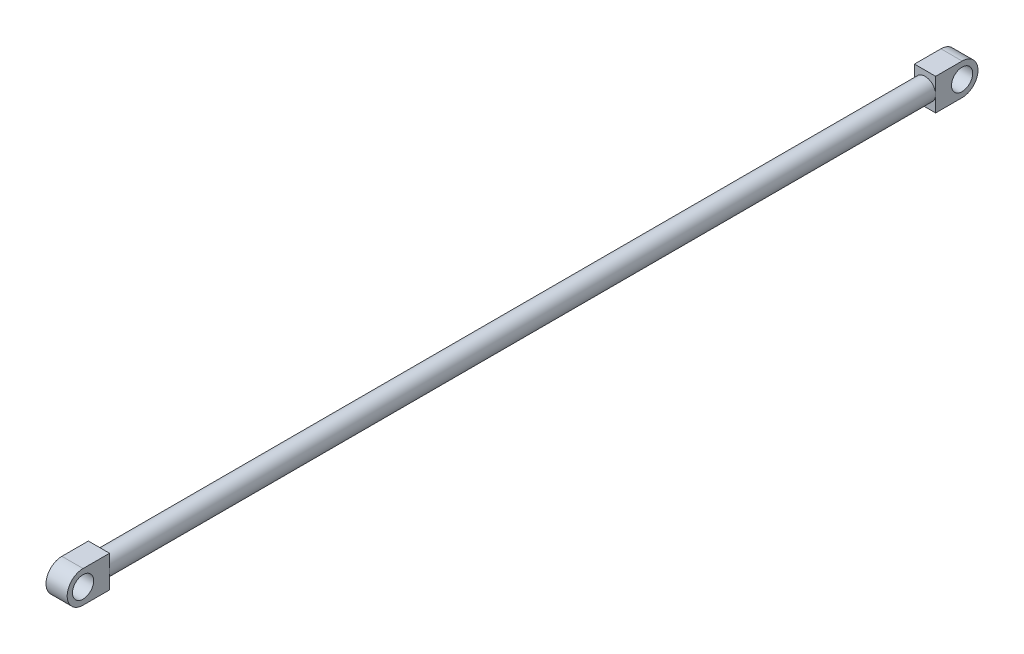
SolidWorks part; units mm, degrees
ref_plane "Front Plane" through (0, 0, 0) normal (0, 0, 1) x (1, 0, 0)
ref_plane "Top Plane" through (0, 0, 0) normal (0, 1, 0) x (1, 0, 0)
ref_plane "Right Plane" through (0, 0, 0) normal (1, 0, 0) x (0, 0, -1)
other "Configuration Table"
sketch "Sketch1" plane through (0, 0, 0) normal (0, 0, 1) x (1, 0, 0)
  circle A0 centre (0, 0) radius 5
  dimension "D1" = 10
extrude "Boss-Extrude1" add sketch "Sketch1" along normal blind 390
sketch "Sketch2" plane through (0, 0, 0) normal (0, 0, -1) x (-1, 0, 0)
  line L1 (-5, 7.5) -> (5, 7.5)
  line L2 (-5, 7.5) -> (-5, -7.5)
  line L3 (-5, -7.5) -> (5, -7.5)
  line L4 (5, 7.5) -> (5, -7.5)
  line L5 (-5, 7.5) -> (5, -7.5) construction
  line L6 (-5, -7.5) -> (5, 7.5) construction
  point P0 (0, 0)
  dimension "D1" = 10
  dimension "D2" = 15
extrude "Boss-Extrude2" add sketch "Sketch2" along normal blind 20
sketch "Sketch3" plane through (0, 0, 390) normal (0, 0, 1) x (1, 0, 0)
  line L1 (-5, -7.5) -> (5, -7.5)
  line L2 (-5, -7.5) -> (-5, 7.5)
  line L3 (-5, 7.5) -> (5, 7.5)
  line L4 (5, -7.5) -> (5, 7.5)
  line L5 (-5, -7.5) -> (5, 7.5) construction
  line L6 (-5, 7.5) -> (5, -7.5) construction
  point P0 (0, 0)
extrude "Boss-Extrude3" add sketch "Sketch3" along normal blind 20
sketch "Sketch4" plane through (5, 0, 0) normal (1, 0, 0) x (0, 0, -1)
  line L0 (-410, -7.5) -> (-410, 7.5) construction
  line L1 (20, 7.5) -> (20, -7.5) construction
  line L2 (12.5, -7.5) -> (27.9572, -19.3446)
  line L3 (27.9572, -19.3446) -> (25.4125, 11.1116)
  line L4 (25.4125, 11.1116) -> (12.5, 7.5)
  line L5 (-402.5, 7.5) -> (-436.593, 16.999)
  line L6 (-436.593, 16.999) -> (-417.5379, -29.4263)
  line L7 (-417.5379, -29.4263) -> (-402.5, -7.5)
  circle A0 centre (12.5, 0) radius 5
  arc A1 (12.5, -7.5) -> (12.5, 7.5) centre (12.5, 0) ccw
  circle A2 centre (-402.5, 0) radius 5
  arc A3 (-402.5, 7.5) -> (-402.5, -7.5) centre (-402.5, 0) ccw
  dimension "D1" = 10
  dimension "D2" = 7.5
  dimension "D3" = 10
  dimension "D4" = 7.5
extrude "Cut-Extrude1" cut sketch "Sketch4" against normal through all
